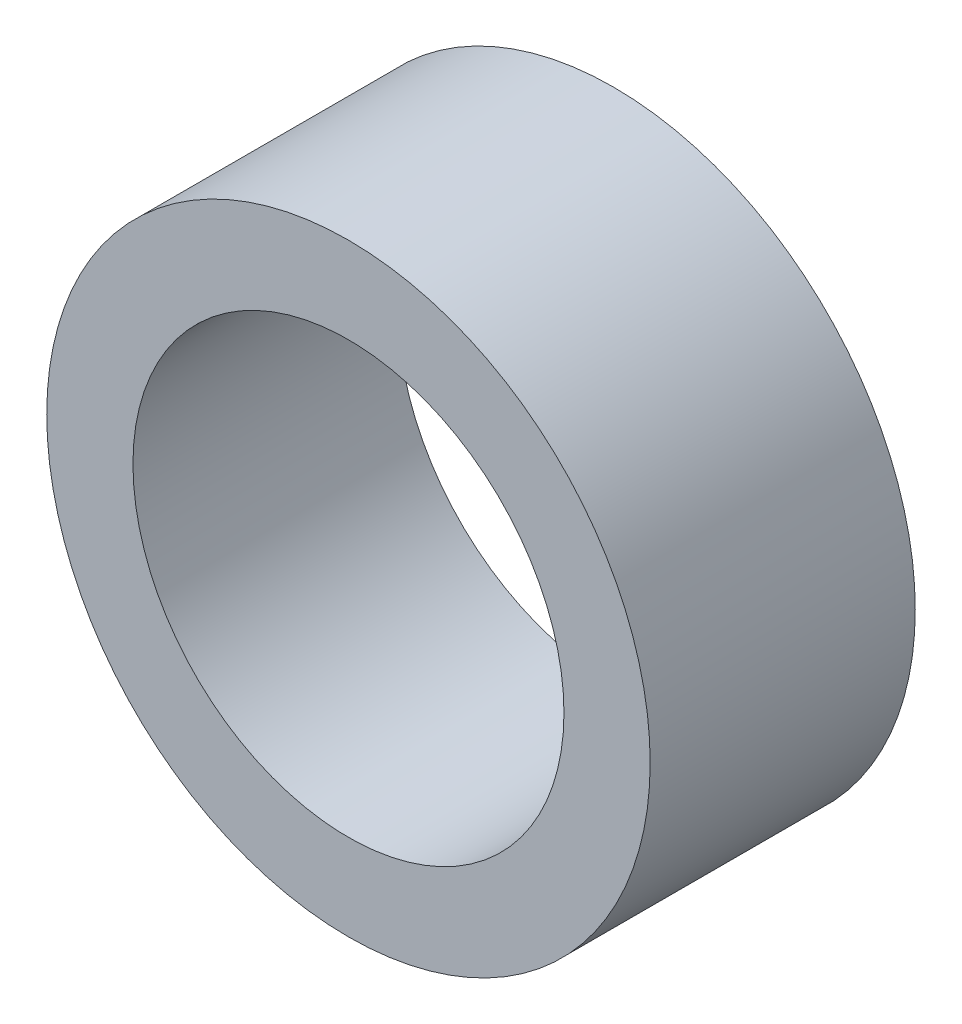
from build123d import *

# Parameters (mm, degrees)
SKETCH_1_R      = 7
SKETCH_1_R_2    = 5
EXTRUDE_1_DEPTH = 6.15


with BuildPart() as part:
    # 草图1 → 凸台-拉伸1 (new body)
    with BuildSketch(Plane.XY):
        Circle(SKETCH_1_R)
        Circle(SKETCH_1_R_2, mode=Mode.SUBTRACT)
    extrude(amount=EXTRUDE_1_DEPTH)


solid = part.part
